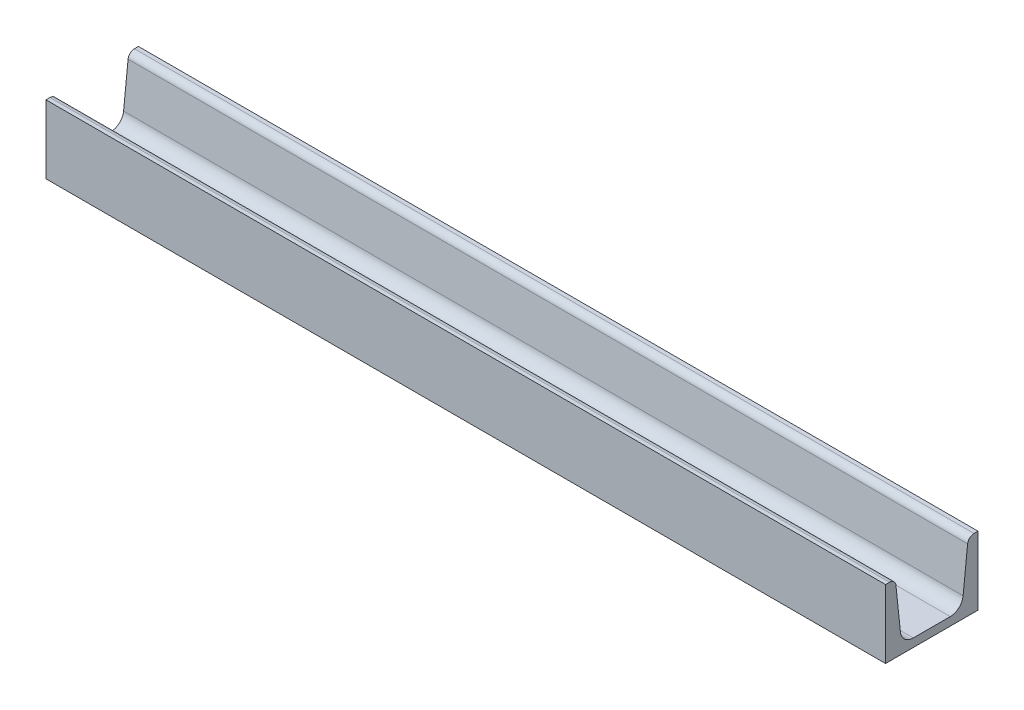
SolidWorks part; units mm, degrees
material "AISI 304"
ref_plane "Front Plane" through (0, 0, 0) normal (0, 0, 1) x (1, 0, 0)
ref_plane "Top Plane" through (0, 0, 0) normal (0, 1, 0) x (1, 0, 0)
ref_plane "Right Plane" through (0, 0, 0) normal (1, 0, 0) x (0, 0, -1)
other "Configuration Table"
sketch "草图1" plane through (0, 0, 0) normal (0, 0, 1) x (1, 0, 0)
  line L0 (-227, 0) -> (227, 0)
  point P4 (0, 0)
  dimension "D1" = 454
other "GB/T 707-1988 hot-rolled channel 05(1)"
ref_plane "Plane1" through (-227, 0, 0) normal (1, 0, 0) x (0, 1, 0)
sketch "Sketch1" plane through (-227, 0, 0) normal (1, 0, 0) x (0, 1, 0)
  line L0 (37, 50) -> (0, 50)
  line L1 (37, 0) -> (0, 0)
  line L2 (0, 50) -> (0, 0)
  line L3 (-9.5694, 25) -> (49.7414, 25) construction
  line L4 (4.5, 34.9892) -> (4.5, 15.0108)
  line L5 (37, 0) -> (37, 2.1406)
  line L6 (37, 50) -> (37, 47.8594)
  line L7 (10.7683, 8.0491) -> (33.8658, 5.6215)
  line L17 (10.7683, 41.9509) -> (33.8658, 44.3785)
  arc A0 (33.8658, 44.3785) -> (37, 47.8594) centre (33.5, 47.8594) ccw
  arc A1 (33.8658, 5.6215) -> (37, 2.1406) centre (33.5, 2.1406) cw
  arc A2 (4.5, 15.0108) -> (10.7683, 8.0491) centre (11.5, 15.0108) ccw
  arc A10 (4.5, 34.9892) -> (10.7683, 41.9509) centre (11.5, 34.9892) cw
  point P6 (0, 0)
  point P8 (0, 25)
  point P9 (4.5, 25.8841)
  point P10 (18.5, 50)
  point P13 (37, 44.7079)
  point P14 (20.75, 43)
  point P19 (4.5, 25)
equation "\"RI@Sketch1\" = \"D1@Sketch1\""
equation "\"D3@Sketch1\" =  ( \"BF@Sketch1\" - \"D6@Sketch1\" )  / 2"
